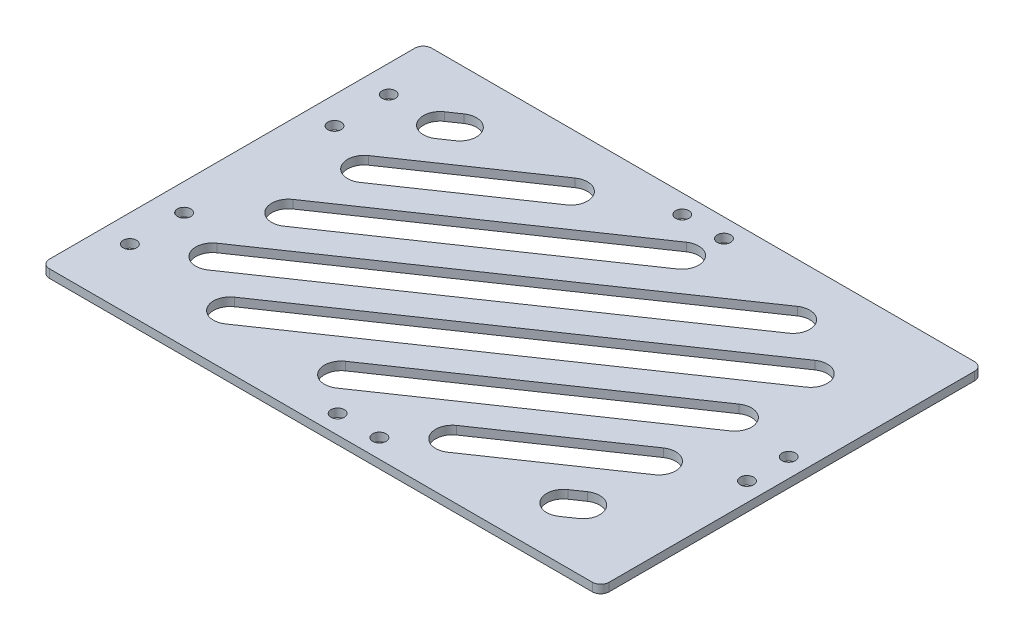
SolidWorks part; units mm, degrees
material "Thornel Mat VMA"
ref_plane "Front Plane" through (0, 0, 0) normal (0, 0, 1) x (1, 0, 0)
ref_plane "Top Plane" through (0, 0, 0) normal (0, 1, 0) x (1, 0, 0)
ref_plane "Right Plane" through (0, 0, 0) normal (1, 0, 0) x (0, 0, -1)
sketch "Sketch1" plane through (0, 0, 0) normal (0, 1, 0) x (1, 0, 0)
  line L0 (-66, 0) -> (68, 0) construction
  line L1 (-66, 45.75) -> (68, 45.75)
  line L2 (-66, 45.75) -> (-66, -45.75)
  line L3 (-66, -45.75) -> (68, -45.75)
  line L4 (68, 45.75) -> (68, -45.75)
  line L5 (0, 45.75) -> (0, -45.75) construction
  line L6 (-59.5, 31) -> (-59.5, 18) construction
  line L7 (-59.5, -31) -> (-59.5, -18) construction
  line L9 (63.5, 3.75) -> (63.5, -6.25) construction
  line L11 (0.5, -41.25) -> (10.5, -41.25) construction
  line L12 (0.5, 41.25) -> (10.5, 41.25) construction
  circle A0 centre (-59.5, 31) radius 1.6
  circle A1 centre (-59.5, 18) radius 1.6
  circle A2 centre (-59.5, -18) radius 1.6
  circle A3 centre (-59.5, -31) radius 1.6
  circle A6 centre (63.5, 3.75) radius 1.6
  circle A7 centre (63.5, -6.25) radius 1.6
  circle A10 centre (0.5, -41.25) radius 1.6
  circle A11 centre (10.5, -41.25) radius 1.6
  circle A12 centre (10.5, 41.25) radius 1.6
  circle A13 centre (0.5, 41.25) radius 1.6
  point P10 (-66, 0)
  dimension "D1" = 3.2
  dimension "D8" = 4.5
  dimension "D9" = 10
  dimension "D12" = 4.5
  dimension "D10" = 3.2
  dimension "D2" = 13
  dimension "D3" = 68
  dimension "D4" = 66
  dimension "D5" = 91.5
  dimension "D6" = 36
  dimension "D7" = 6.5
  dimension "D11" = 39.5
  dimension "D15" = 57.5
extrude "Boss-Extrude1" add sketch "Sketch1" along normal blind 2
sketch "Team emblem" [suppressed] plane through (0, 2, 0) normal (0, 1, 0) x (1, 0, 0)
  line L0 (-25, 38) -> (-25, -22) construction
  line L1 (-12.515, 33.7) -> (-12.515, 35.2787)
  line L2 (-37.485, 33.7) -> (-37.485, 35.2787)
  line L3 (-33.13, 16.8019) -> (-33.13, 11.5819)
  line L4 (-33.13, 11.5819) -> (-34.702, 9.9305)
  line L5 (-34.702, 9.9305) -> (-36.3011, 4.7584)
  line L6 (-33.4579, 3.2225) -> (-31.1856, 10.5724)
  line L7 (-16.5421, 3.2225) -> (-18.8144, 10.5724)
  line L8 (-17.5104, 17.0865) -> (-13.6989, 4.7584)
  line L9 (-21.0663, 32.392) -> (-19.6973, 32.769)
  line L10 (-19.6973, 32.769) -> (-18.0096, 33.5704)
  line L11 (-18.0096, 33.5704) -> (-17.8613, 32.2487)
  line L12 (-18.4024, 35.9034) -> (-17.7524, 35.7605)
  line L13 (-6.1254, -12) -> (-2.6393, -12)
  line L14 (-43.8746, -12) -> (-47.3607, -12)
  arc A0 (-16.6314, -20.8091) -> (-2.6393, -12) centre (-25, 8) ccw
  arc A2 (-33.3686, -20.8091) -> (-33.13, 16.8019) centre (-24.3625, -2.06) cw
  arc A3 (-16.6314, -20.8091) -> (-17.5104, 17.0865) centre (-25.6375, -2.06) ccw
  arc A4 (-19.8705, 26.2753) -> (-12.515, 33.7) centre (-19.94, 33.7) ccw
  arc A5 (-30.1295, 26.2753) -> (-37.485, 33.7) centre (-30.06, 33.7) cw
  arc A6 (-47.3607, -12) -> (-33.3686, -20.8091) centre (-25, 8) ccw
  arc A7 (-36.3011, 4.7584) -> (-33.4579, 3.2225) centre (-25, 22.28) ccw
  arc A9 (-32.1188, 2.6829) -> (-31.1856, 10.5724) centre (-66.67, 10.77) ccw
  arc A10 (-32.1188, 2.6829) -> (-29.0372, 1.8246) centre (-25, 22.28) ccw
  arc A12 (-27.4096, 1.5697) -> (-27.9405, 8.9327) centre (-66.67, 2.44) ccw
  arc A13 (-29.0372, 1.8246) -> (-27.9405, 8.9327) centre (-66.67, 11.27) ccw
  arc A14 (-27.4096, 1.5697) -> (-22.5904, 1.5697) centre (-25, 22.28) ccw
  arc A15 (-22.5904, 1.5697) -> (-22.0595, 8.9327) centre (16.67, 2.44) cw
  arc A16 (-20.9628, 1.8246) -> (-22.0595, 8.9327) centre (16.67, 11.27) cw
  arc A17 (-30.1295, 26.2753) -> (-28.9744, 32.0412) centre (-66.7, 36.6) ccw
  arc A18 (-17.8812, 2.6829) -> (-18.8144, 10.5724) centre (16.67, 10.77) cw
  arc A19 (-19.8705, 26.2753) -> (-21.0663, 32.392) centre (16.7, 36.6) cw
  arc A20 (-20.9628, 1.8246) -> (-17.8812, 2.6829) centre (-25, 22.28) ccw
  arc A21 (-16.5421, 3.2225) -> (-13.6989, 4.7584) centre (-25, 22.28) ccw
  arc A22 (-20.8, 36.4498) -> (-31.4255, 34.2262) centre (-21.93, 15.35) ccw
  arc A23 (-16.5042, 35.0804) -> (-17.7524, 35.7605) centre (-18.3, 33.27) ccw
  arc A25 (-17.8613, 32.2487) -> (-16.5042, 35.0804) centre (-18.3, 34.2) ccw
  arc A29 (-6.1077, 27.9833) -> (-12.515, 35.2787) centre (-17.46, 24.4743) ccw
  arc A30 (-2.2672, 23.4748) -> (-0.7491, 25.6605) centre (-25, 40.8837) ccw
  arc A31 (-6.1077, 27.9833) -> (-5.5019, 30.7996) centre (-25, 33.5203) ccw
  arc A32 (-2.2672, 23.4748) -> (-5.5019, 30.7996) centre (-11.5161, 23.767) ccw
  arc A33 (1.6644, 14.7277) -> (3.8374, 16.2708) centre (-25, 54.5789) ccw
  arc A34 (1.6644, 14.7277) -> (-0.7491, 25.6605) centre (-12.0455, 17.434) ccw
  arc A35 (2.163, 3.7077) -> (4.8783, 5.3) centre (-25, 53.1378) ccw
  arc A36 (2.163, 3.7077) -> (3.8374, 16.2708) centre (-11.3811, 11.906) ccw
  arc A37 (-1.1678, -5.7213) -> (1.8513, -5.3793) centre (-25, 218.1341) ccw
  arc A38 (-1.1678, -5.7213) -> (4.8783, 5.3) centre (-10.7675, 6.7139) ccw
  arc A40 (-6.1254, -12) -> (1.8513, -5.3793) centre (-9.635, 0.344) ccw
  circle A41 centre (-25, 8) radius 27.5 construction
  arc A42 (-43.8923, 27.9833) -> (-44.4981, 30.7996) centre (-25, 33.5203) cw
  arc A43 (-43.8923, 27.9833) -> (-37.485, 35.2787) centre (-32.54, 24.4743) cw
  arc A44 (-47.7328, 23.4748) -> (-44.4981, 30.7996) centre (-38.4839, 23.767) cw
  arc A45 (-47.7328, 23.4748) -> (-49.2509, 25.6605) centre (-25, 40.8837) cw
  arc A46 (-51.6644, 14.7277) -> (-49.2509, 25.6605) centre (-37.9545, 17.434) cw
  arc A47 (-51.6644, 14.7277) -> (-53.8374, 16.2708) centre (-25, 54.5789) cw
  arc A48 (-52.163, 3.7077) -> (-53.8374, 16.2708) centre (-38.6189, 11.906) cw
  arc A49 (-52.163, 3.7077) -> (-54.8783, 5.3) centre (-25, 53.1378) cw
  arc A50 (-48.8322, -5.7213) -> (-54.8783, 5.3) centre (-39.2325, 6.7139) cw
  arc A51 (-48.8322, -5.7213) -> (-51.8513, -5.3793) centre (-25, 218.1341) cw
  arc A52 (-43.8746, -12) -> (-51.8513, -5.3793) centre (-40.365, 0.344) cw
  arc A53 (-28.9744, 32.0412) -> (-31.4255, 34.2262) centre (-30.96, 32.2812) ccw
  spline S0 degree 3 poles (-20.8, 36.4498) (-20.2858, 35.8279) (-18.8685, 36.0059) (-18.4024, 35.9034) knots 0 0 0 0 1 1 1 1
  spline S1 degree 3 poles (-22.2858, 34.0584) (-22.7796, 35.9592) (-21.5435, 34.6039) (-20.1915, 35.1653) (-20.9556, 33.6368) (-22.2858, 34.0584) (-22.7796, 35.9592) (-21.5435, 34.6039) knots -0.60913 -0.442651 -0.194324 0 0.241967 0.39087 0.557349 0.805676 1 1.241967 1.39087 1.557349 only from (-22.5, 35.3861) to (-22.5, 35.3861)
  dimension "D1" = 60
  dimension "D2" = 20.8
  dimension "D5" = 25.7
  dimension "D7" = 7.425
  dimension "D8" = 41.7
  dimension "D16" = 35.485
  dimension "D19" = 39.27
  dimension "D21" = 0.5
  dimension "D22" = 38.8
  dimension "D23" = 41.7
  dimension "D25" = 55
  dimension "D26" = 7.35
  dimension "D28" = 21.13
  dimension "D29" = 25.27
  dimension "D31" = 0.93
  dimension "D32" = 2
  dimension "D33" = 5.1
  dimension "D41" = 8
  dimension "D42" = 9.59
  dimension "D44" = 7
  dimension "D46" = 10
  dimension "D48" = 20
  dimension "D49" = 11.1
  dimension "D43" = 11.02
  dimension "D47" = 8
  dimension "D52" = 38
  dimension "D57" = 2
  dimension "D3" = 10.06
  dimension "D4" = 1.275
  dimension "D6" = 10.12
  dimension "D9" = 14.28
  dimension "D10" = 8.13
  dimension "D11" = 5.22
  dimension "D12" = 136.41
  dimension "D13" = 2.28
  dimension "D14" = 17.18
  dimension "D15" = 3.17
  dimension "D17" = 41.67
  dimension "D18" = 2.77
  dimension "D20" = 8.33
  dimension "D24" = 28.6
  dimension "D27" = 3.07
  dimension "D30" = 6.7
  dimension "D34" = 74.6
  dimension "D35" = 1.42
  dimension "D36" = 170
  dimension "D37" = 71
  dimension "D38" = 1.33
  dimension "D39" = 0.65
  dimension "D40" = 77.6
  dimension "D45" = 7.54
  dimension "D50" = 11.02
  dimension "D51" = 10.45
  dimension "D53" = 4.8
  dimension "D54" = 28.5
  dimension "D55" = 4.2
  dimension "D56" = 90
  dimension "D58" = 5.96
  dimension "D59" = 2.5
  dimension "D60" = 2
  dimension "D61" = 0.5
  dimension "D62" = 1.2
  dimension "D63" = 0.3
  dimension "D64" = 0.4
  dimension "D65" = 1
  dimension "D66" = 0.8
  dimension "D67" = 8
  dimension "D68" = 25
sketch "Sketch4" [suppressed] plane through (0, 2, 0) normal (0, 1, 0) x (1, 0, 0)
  line L0 (-25, 42) -> (-25, -26) construction
  line L3 (-27.5, 41.908) -> (-27.5, 35.7326)
  line L8 (-22.5, 41.908) -> (-22.5, 36.4723)
  line L9 (6.4758, 20.8558) -> (1.7989, 19.3361)
  line L10 (8.0209, 16.1005) -> (4.1747, 14.8508)
  line L11 (-3.0469, -17.9627) -> (-5.4052, -14.7166)
  line L12 (-7.0919, -20.9016) -> (-9.4503, -17.6556)
  line L13 (-42.9081, -20.9016) -> (-40.5497, -17.6556)
  line L42 (-46.9531, -17.9627) -> (-44.5948, -14.7166)
  line L43 (-58.0209, 16.1005) -> (-54.1747, 14.8508)
  line L44 (-56.4758, 20.8558) -> (-51.7989, 19.3361)
  line L45 (-43.3105, 6.5198) -> (-49.4142, 0.4161)
  line L46 (-44.7, 2.3019) -> (-48, -0.9981)
  line L48 (-43.8746, -12) -> (-47.3607, -12)
  line L49 (-33.13, 16.8019) -> (-33.13, 11.5819)
  line L50 (-33.13, 11.5819) -> (-34.702, 9.9305)
  line L51 (-34.702, 9.9305) -> (-36.3011, 4.7584)
  line L52 (-33.4579, 3.2225) -> (-31.1856, 10.5724)
  line L53 (-18.8144, 10.5724) -> (-16.5421, 3.2225)
  line L54 (-13.6989, 4.7584) -> (-17.5104, 17.0865)
  line L55 (-2.6393, -12) -> (-6.1254, -12)
  line L56 (-12.515, 35.2787) -> (-12.515, 33.7)
  line L57 (-21.0663, 32.392) -> (-19.6973, 32.769)
  line L58 (-19.6973, 32.769) -> (-18.0096, 33.5704)
  line L59 (-18.0096, 33.5704) -> (-17.8613, 32.2487)
  line L60 (-17.7524, 35.7605) -> (-18.4024, 35.9034)
  line L61 (-37.485, 33.7) -> (-37.485, 35.2787)
  line L62 (-43.8746, -12) -> (-47.3607, -12)
  line L63 (-33.13, 16.8019) -> (-33.13, 11.5819)
  line L64 (-33.13, 11.5819) -> (-34.702, 9.9305)
  line L65 (-34.702, 9.9305) -> (-36.3011, 4.7584)
  line L66 (-33.4579, 3.2225) -> (-31.1856, 10.5724)
  line L67 (-18.8144, 10.5724) -> (-16.5421, 3.2225)
  line L68 (-13.6989, 4.7584) -> (-17.5104, 17.0865)
  line L69 (-2.6393, -12) -> (-6.1254, -12)
  line L70 (-12.515, 35.2787) -> (-12.515, 33.7)
  line L71 (-21.0663, 32.392) -> (-19.6973, 32.769)
  line L72 (-19.6973, 32.769) -> (-18.0096, 33.5704)
  line L73 (-18.0096, 33.5704) -> (-17.8613, 32.2487)
  line L74 (-17.7524, 35.7605) -> (-18.4024, 35.9034)
  line L75 (-37.485, 33.7) -> (-37.485, 35.2787)
  line L77 (-49.4142, 0.4161) -> (-48, -0.9981)
  line L78 (-44.8311, 21.2627) -> (-36.3458, 29.7479) construction
  line L79 (-54.0846, 8.5198) -> (-50.5029, 8.5198)
  line L80 (-50.5029, 8.5198) -> (-36.2226, 22.8001)
  line L81 (-53.5066, 6.5198) -> (-49.6745, 6.5198)
  line L82 (-49.6745, 6.5198) -> (-34.8084, 21.3859)
  line L83 (-44.5227, 22.9853) -> (-36.8384, 30.6696)
  line L84 (-43.1085, 21.5711) -> (-35.7499, 28.9297)
  arc A6 (-27.5, 41.908) -> (-56.4758, 20.8558) centre (-25, 8) ccw
  arc A7 (-27.5, 35.7326) -> (-31.4255, 34.2262) centre (-21.93, 15.35) ccw
  arc A8 (-42.9081, -20.9016) -> (-7.0919, -20.9016) centre (-25, 8) ccw
  arc A9 (-40.5497, -17.6556) -> (-33.3686, -20.8091) centre (-25, 8) ccw
  arc A10 (-3.0469, -17.9627) -> (8.0209, 16.1005) centre (-25, 8) ccw
  arc A11 (-5.4052, -14.7166) -> (-2.6393, -12) centre (-25, 8) ccw
  arc A12 (6.4758, 20.8558) -> (-22.5, 41.908) centre (-25, 8) ccw
  arc A13 (-58.0209, 16.1005) -> (-46.9531, -17.9627) centre (-25, 8) ccw
  arc A15 (-44.7, 2.3019) -> (-33.3686, -20.8091) centre (-24.3625, -2.06) ccw
  arc A18 (-34.8084, 21.3859) -> (-36.2226, 22.8001) centre (-34.5, 23.1085) ccw
  arc A19 (-53.5066, 6.5198) -> (-52.163, 3.7077) centre (-38.6189, 11.906) ccw
  arc A20 (-44.5227, 22.9853) -> (-43.1085, 21.5711) centre (-44.8311, 21.2627) ccw
  arc A21 (-35.7499, 28.9297) -> (-30.1295, 26.2753) centre (-30.06, 33.7) ccw
  arc A135 (-47.3607, -12) -> (-33.3686, -20.8091) centre (-25, 8) ccw
  arc A136 (-33.13, 16.8019) -> (-33.3686, -20.8091) centre (-24.3625, -2.06) ccw
  arc A137 (-36.3011, 4.7584) -> (-33.4579, 3.2225) centre (-25, 22.28) ccw
  arc A138 (-32.1188, 2.6829) -> (-31.1856, 10.5724) centre (-66.67, 10.77) ccw
  arc A139 (-32.1188, 2.6829) -> (-29.0372, 1.8246) centre (-25, 22.28) ccw
  arc A140 (-29.0372, 1.8246) -> (-27.9405, 8.9327) centre (-66.67, 11.27) ccw
  arc A141 (-27.4096, 1.5697) -> (-27.9405, 8.9327) centre (-66.67, 2.44) ccw
  arc A142 (-27.4096, 1.5697) -> (-22.5904, 1.5697) centre (-25, 22.28) ccw
  arc A143 (-22.0595, 8.9327) -> (-22.5904, 1.5697) centre (16.67, 2.44) ccw
  arc A144 (-22.0595, 8.9327) -> (-20.9628, 1.8246) centre (16.67, 11.27) ccw
  arc A145 (-20.9628, 1.8246) -> (-17.8812, 2.6829) centre (-25, 22.28) ccw
  arc A146 (-18.8144, 10.5724) -> (-17.8812, 2.6829) centre (16.67, 10.77) ccw
  arc A147 (-16.5421, 3.2225) -> (-13.6989, 4.7584) centre (-25, 22.28) ccw
  arc A148 (-16.6314, -20.8091) -> (-17.5104, 17.0865) centre (-25.6375, -2.06) ccw
  arc A149 (-16.6314, -20.8091) -> (-2.6393, -12) centre (-25, 8) ccw
  arc A150 (-6.1254, -12) -> (1.8513, -5.3793) centre (-9.635, 0.344) ccw
  arc A151 (-1.1678, -5.7213) -> (1.8513, -5.3793) centre (-25, 218.1341) ccw
  arc A152 (-1.1678, -5.7213) -> (4.8783, 5.3) centre (-10.7675, 6.7139) ccw
  arc A153 (2.163, 3.7077) -> (4.8783, 5.3) centre (-25, 53.1378) ccw
  arc A154 (2.163, 3.7077) -> (3.8374, 16.2708) centre (-11.3811, 11.906) ccw
  arc A155 (1.6644, 14.7277) -> (3.8374, 16.2708) centre (-25, 54.5789) ccw
  arc A156 (1.6644, 14.7277) -> (-0.7491, 25.6605) centre (-12.0455, 17.434) ccw
  arc A157 (-2.2672, 23.4748) -> (-0.7491, 25.6605) centre (-25, 40.8837) ccw
  arc A158 (-2.2672, 23.4748) -> (-5.5019, 30.7996) centre (-11.5161, 23.767) ccw
  arc A159 (-6.1077, 27.9833) -> (-5.5019, 30.7996) centre (-25, 33.5203) ccw
  arc A160 (-6.1077, 27.9833) -> (-12.515, 35.2787) centre (-17.46, 24.4743) ccw
  arc A161 (-19.8705, 26.2753) -> (-12.515, 33.7) centre (-19.94, 33.7) ccw
  arc A162 (-21.0663, 32.392) -> (-19.8705, 26.2753) centre (16.7, 36.6) ccw
  arc A163 (-17.8613, 32.2487) -> (-16.5042, 35.0804) centre (-18.3, 34.2) ccw
  arc A164 (-16.5042, 35.0804) -> (-17.7524, 35.7605) centre (-18.3, 33.27) ccw
  arc A165 (-20.8, 36.4498) -> (-31.4255, 34.2262) centre (-21.93, 15.35) ccw
  arc A166 (-30.1295, 26.2753) -> (-28.9744, 32.0412) centre (-66.7, 36.6) ccw
  arc A167 (-37.485, 33.7) -> (-30.1295, 26.2753) centre (-30.06, 33.7) ccw
  arc A168 (-37.485, 35.2787) -> (-43.8923, 27.9833) centre (-32.54, 24.4743) ccw
  arc A169 (-44.4981, 30.7996) -> (-43.8923, 27.9833) centre (-25, 33.5203) ccw
  arc A170 (-44.4981, 30.7996) -> (-47.7328, 23.4748) centre (-38.4839, 23.767) ccw
  arc A171 (-49.2509, 25.6605) -> (-47.7328, 23.4748) centre (-25, 40.8837) ccw
  arc A172 (-49.2509, 25.6605) -> (-51.6644, 14.7277) centre (-37.9545, 17.434) ccw
  arc A173 (-53.8374, 16.2708) -> (-51.6644, 14.7277) centre (-25, 54.5789) ccw
  arc A174 (-53.8374, 16.2708) -> (-52.163, 3.7077) centre (-38.6189, 11.906) ccw
  arc A175 (-54.8783, 5.3) -> (-52.163, 3.7077) centre (-25, 53.1378) ccw
  arc A176 (-54.8783, 5.3) -> (-48.8322, -5.7213) centre (-39.2325, 6.7139) ccw
  arc A177 (-51.8513, -5.3793) -> (-48.8322, -5.7213) centre (-25, 218.1341) ccw
  arc A178 (-51.8513, -5.3793) -> (-43.8746, -12) centre (-40.365, 0.344) ccw
  arc A179 (-47.3607, -12) -> (-44.5948, -14.7166) centre (-25, 8) ccw
  arc A180 (-33.13, 16.8019) -> (-43.3105, 6.5198) centre (-24.3625, -2.06) ccw
  arc A181 (-36.3011, 4.7584) -> (-33.4579, 3.2225) centre (-25, 22.28) ccw
  arc A182 (-32.1188, 2.6829) -> (-31.1856, 10.5724) centre (-66.67, 10.77) ccw
  arc A183 (-32.1188, 2.6829) -> (-29.0372, 1.8246) centre (-25, 22.28) ccw
  arc A184 (-29.0372, 1.8246) -> (-27.9405, 8.9327) centre (-66.67, 11.27) ccw
  arc A185 (-27.4096, 1.5697) -> (-27.9405, 8.9327) centre (-66.67, 2.44) ccw
  arc A186 (-27.4096, 1.5697) -> (-22.5904, 1.5697) centre (-25, 22.28) ccw
  arc A187 (-22.0595, 8.9327) -> (-22.5904, 1.5697) centre (16.67, 2.44) ccw
  arc A188 (-22.0595, 8.9327) -> (-20.9628, 1.8246) centre (16.67, 11.27) ccw
  arc A189 (-20.9628, 1.8246) -> (-17.8812, 2.6829) centre (-25, 22.28) ccw
  arc A190 (-18.8144, 10.5724) -> (-17.8812, 2.6829) centre (16.67, 10.77) ccw
  arc A191 (-16.5421, 3.2225) -> (-13.6989, 4.7584) centre (-25, 22.28) ccw
  arc A192 (-16.6314, -20.8091) -> (-17.5104, 17.0865) centre (-25.6375, -2.06) ccw
  arc A193 (-16.6314, -20.8091) -> (-9.4503, -17.6556) centre (-25, 8) ccw
  arc A194 (-6.1254, -12) -> (1.8513, -5.3793) centre (-9.635, 0.344) ccw
  arc A195 (-1.1678, -5.7213) -> (1.8513, -5.3793) centre (-25, 218.1341) ccw
  arc A196 (-1.1678, -5.7213) -> (4.8783, 5.3) centre (-10.7675, 6.7139) ccw
  arc A197 (2.163, 3.7077) -> (4.8783, 5.3) centre (-25, 53.1378) ccw
  arc A198 (2.163, 3.7077) -> (4.1747, 14.8508) centre (-11.3811, 11.906) ccw
  arc A200 (1.7989, 19.3361) -> (-0.7491, 25.6605) centre (-12.0455, 17.434) ccw
  arc A201 (-2.2672, 23.4748) -> (-0.7491, 25.6605) centre (-25, 40.8837) ccw
  arc A202 (-2.2672, 23.4748) -> (-5.5019, 30.7996) centre (-11.5161, 23.767) ccw
  arc A203 (-6.1077, 27.9833) -> (-5.5019, 30.7996) centre (-25, 33.5203) ccw
  arc A204 (-6.1077, 27.9833) -> (-12.515, 35.2787) centre (-17.46, 24.4743) ccw
  arc A205 (-19.8705, 26.2753) -> (-12.515, 33.7) centre (-19.94, 33.7) ccw
  arc A206 (-21.0663, 32.392) -> (-19.8705, 26.2753) centre (16.7, 36.6) ccw
  arc A207 (-17.8613, 32.2487) -> (-16.5042, 35.0804) centre (-18.3, 34.2) ccw
  arc A208 (-16.5042, 35.0804) -> (-17.7524, 35.7605) centre (-18.3, 33.27) ccw
  arc A209 (-20.8, 36.4498) -> (-22.5, 36.4723) centre (-21.93, 15.35) ccw
  arc A210 (-30.1295, 26.2753) -> (-28.9744, 32.0412) centre (-66.7, 36.6) ccw
  arc A211 (-37.485, 33.7) -> (-36.8384, 30.6696) centre (-30.06, 33.7) ccw
  arc A212 (-37.485, 35.2787) -> (-43.8923, 27.9833) centre (-32.54, 24.4743) ccw
  arc A213 (-44.4981, 30.7996) -> (-43.8923, 27.9833) centre (-25, 33.5203) ccw
  arc A214 (-44.4981, 30.7996) -> (-47.7328, 23.4748) centre (-38.4839, 23.767) ccw
  arc A215 (-49.2509, 25.6605) -> (-47.7328, 23.4748) centre (-25, 40.8837) ccw
  arc A216 (-49.2509, 25.6605) -> (-51.7989, 19.3361) centre (-37.9545, 17.434) ccw
  arc A218 (-54.1747, 14.8508) -> (-54.0846, 8.5198) centre (-38.6189, 11.906) ccw
  arc A219 (-54.8783, 5.3) -> (-52.163, 3.7077) centre (-25, 53.1378) ccw
  arc A220 (-54.8783, 5.3) -> (-48.8322, -5.7213) centre (-39.2325, 6.7139) ccw
  arc A221 (-51.8513, -5.3793) -> (-48.8322, -5.7213) centre (-25, 218.1341) ccw
  arc A222 (-51.8513, -5.3793) -> (-43.8746, -12) centre (-40.365, 0.344) ccw
  arc A232 (-28.9744, 32.0412) -> (-31.4255, 34.2262) centre (-30.96, 32.2812) ccw
  arc A233 (-28.9744, 32.0412) -> (-31.4255, 34.2262) centre (-30.96, 32.2812) ccw
  spline S0 degree 3 poles (-21.5435, 34.6039) (-22.7796, 35.9592) (-22.2858, 34.0584) (-20.9556, 33.6368) (-20.1915, 35.1653) (-21.5435, 34.6039) (-22.7796, 35.9592) (-22.2858, 34.0584) knots -0.557349 -0.39087 -0.241967 0 0.194324 0.442651 0.60913 0.758033 1 1.194324 1.442651 1.60913 only from (-22.5, 35.3861) to (-22.5, 35.3861) construction
  spline S1 degree 3 poles (-1772.4748, -924.8076) (1747.4533, 1033.1302) (-1763.0741, -1000.2366) (1663.8646, 1113.8816) knots -9.353839 -9.353839 -9.353839 -9.353839 10.249272 10.249272 10.249272 10.249272 only from (-18.4024, 35.9034) to (-20.8, 36.4498)
  spline S2 degree 3 poles (-18.4024, 35.9034) (-18.8685, 36.0059) (-20.2858, 35.8279) (-20.8, 36.4498) knots 0 0 0 0 1 1 1 1
  spline S3 degree 3 poles (-21.5435, 34.6039) (-22.7796, 35.9592) (-22.2858, 34.0584) (-20.9556, 33.6368) (-20.1915, 35.1653) (-21.5435, 34.6039) (-22.7796, 35.9592) (-22.2858, 34.0584) knots -0.557349 -0.39087 -0.241967 0 0.194324 0.442651 0.60913 0.758033 1 1.194324 1.442651 1.60913 only from (-22.5, 35.3861) to (-22.5, 35.3861)
  point P86 (-25, 8)
  dimension "D2" = 4
  dimension "D4" = 5
  dimension "D5" = 1.75
  dimension "D8" = 2
  dimension "D12" = 2
  dimension "D14" = 1
  dimension "D3" = 5
  dimension "D6" = 2
  dimension "D7" = 45
  dimension "D9" = 4
  dimension "D10" = 19.7
  dimension "D11" = 23
  dimension "D13" = 2
  dimension "D15" = 12
  dimension "D16" = 9.5
  dimension "D17" = 4.5
  dimension "D21" = 8
  dimension "D1" = 0
extrude "Cut-Extrude1" [suppressed] cut sketch "Sketch4" against normal through all contours A210 A233 A7 L3 A6 L44 A216 A215 A214 A213 A212 L75 A211 | S2 L74 A208 A207 L73 L72 L71 A206 A205 L70 A204 A203 A202 A201 A200 L9 A12 L8 A209 | A222 A221 A220 A219 A218 L43 A13 L42 A179 L62 | L0 A186 A185 A184 A183 A182 L66 A181 L65 L64 L63 A180 A9 L13 A8 | A186 L0 A8 L12 A193 A192 L68 A191 L67 A190 A189 A188 A187 | A198 A197 A196 A195 A194 L69 A11 L11 A10 L10 | S3
fillet "R0.5 Fillet 1" [suppressed] radius 0.5
fillet "R0.5 Fillet 2" [suppressed] radius 0.5
fillet "R2 Fillet 3" [suppressed] radius 2
sketch "Sketch5" plane through (0, 2, 0) normal (0, 1, 0) x (1, 0, 0)
  line L0 (-66, -45.75) -> (68, 45.75) construction
  line L1 (-47, 30.7958) -> (-44.2163, 32.6966) construction
  line L2 (-49.2556, 34.0992) -> (-46.472, 36)
  line L3 (-44.7444, 27.4925) -> (-41.9607, 29.3933)
  line L4 (-47, 12.6324) -> (-17.6163, 32.6966) construction
  line L5 (-49.2556, 15.9358) -> (-19.872, 36)
  line L6 (-44.7444, 9.3291) -> (-15.3607, 29.3933)
  line L7 (-47, -5.531) -> (8.9836, 32.6966) construction
  line L8 (-49.2556, -2.2277) -> (6.728, 36)
  line L9 (-44.7444, -8.8343) -> (11.2393, 29.3933)
  line L10 (-47, -23.6944) -> (35.5836, 32.6966) construction
  line L11 (-49.2556, -20.3911) -> (33.328, 36)
  line L12 (-44.7444, -26.9978) -> (37.8392, 29.3933)
  line L13 (-33.7, -32.7761) -> (48.8836, 23.6149) construction
  line L14 (-66.1164, 45.75) -> (68, -45.8295) construction
  line L15 (-35.9557, -29.4728) -> (46.6279, 26.9183)
  line L16 (-31.4444, -36.0795) -> (51.1392, 20.3116)
  line L17 (-7.1, -32.7761) -> (48.8836, 5.4515) construction
  line L18 (-9.3557, -29.4728) -> (46.6279, 8.7549)
  line L19 (-4.8444, -36.0795) -> (51.1392, 2.1482)
  line L20 (19.4999, -32.7761) -> (48.8836, -12.7119) construction
  line L21 (17.2443, -29.4728) -> (46.6279, -9.4086)
  line L22 (21.7556, -36.0795) -> (51.1392, -16.0153)
  line L23 (46.0999, -32.7761) -> (48.8836, -30.8753) construction
  line L24 (43.8443, -29.4728) -> (46.6279, -27.572)
  line L25 (48.3555, -36.0795) -> (51.1392, -34.1787)
  line L26 (-66, 45.75) -> (68, -45.75) construction
  line L27 (68, 45.75) -> (-66, 45.75) construction
  line L28 (68, -45.75) -> (68, 45.75) construction
  arc A0 (-49.2556, 34.0992) -> (-44.7444, 27.4925) centre (-47, 30.7958) ccw
  arc A1 (-41.9607, 29.3933) -> (-46.472, 36) centre (-44.2163, 32.6966) ccw
  arc A2 (-49.2556, 15.9358) -> (-44.7444, 9.3291) centre (-47, 12.6324) ccw
  arc A3 (-15.3607, 29.3933) -> (-19.872, 36) centre (-17.6163, 32.6966) ccw
  arc A4 (-49.2556, -2.2277) -> (-44.7444, -8.8343) centre (-47, -5.531) ccw
  arc A5 (11.2393, 29.3933) -> (6.728, 36) centre (8.9836, 32.6966) ccw
  arc A6 (-49.2556, -20.3911) -> (-44.7444, -26.9978) centre (-47, -23.6944) ccw
  arc A7 (37.8392, 29.3933) -> (33.328, 36) centre (35.5836, 32.6966) ccw
  arc A8 (-35.9557, -29.4728) -> (-31.4444, -36.0795) centre (-33.7, -32.7761) ccw
  arc A9 (51.1392, 20.3116) -> (46.6279, 26.9183) centre (48.8836, 23.6149) ccw
  arc A10 (-9.3557, -29.4728) -> (-4.8444, -36.0795) centre (-7.1, -32.7761) ccw
  arc A11 (51.1392, 2.1482) -> (46.6279, 8.7549) centre (48.8836, 5.4515) ccw
  arc A12 (17.2443, -29.4728) -> (21.7556, -36.0795) centre (19.4999, -32.7761) ccw
  arc A13 (51.1392, -16.0153) -> (46.6279, -9.4086) centre (48.8836, -12.7119) ccw
  arc A14 (43.8443, -29.4728) -> (48.3555, -36.0795) centre (46.0999, -32.7761) ccw
  arc A15 (51.1392, -34.1787) -> (46.6279, -27.572) centre (48.8836, -30.8753) ccw
  circle A16 centre (-59.5, -18) radius 1.6 construction
  point P6 (-45.6082, 31.7462)
  point P12 (-32.3082, 22.6645)
  point P19 (-19.0082, 13.5828)
  point P26 (-5.7082, 4.5011)
  point P33 (7.5918, -4.5806)
  point P44 (20.8918, -13.6623)
  point P51 (34.1918, -22.744)
  point P58 (47.4917, -31.8257)
  dimension "D1" = 4
  dimension "D2" = 7
  dimension "D3" = 3.5
  dimension "D4" = 7
  dimension "D5" = 7
  dimension "D6" = 7
  dimension "D7" = 7
  dimension "D8" = 7
  dimension "D9" = 7
  dimension "D10" = 100
  dimension "D11" = 12.5
extrude "Cut-Extrude2" cut sketch "Sketch5" against normal through all and the other way through all
fillet "R2 Fillet 1" radius 2 4 edges at (-66, 1, -45.75) (68, 1, -45.75) (68, 1, 45.75) (-66, 1, 45.75)
